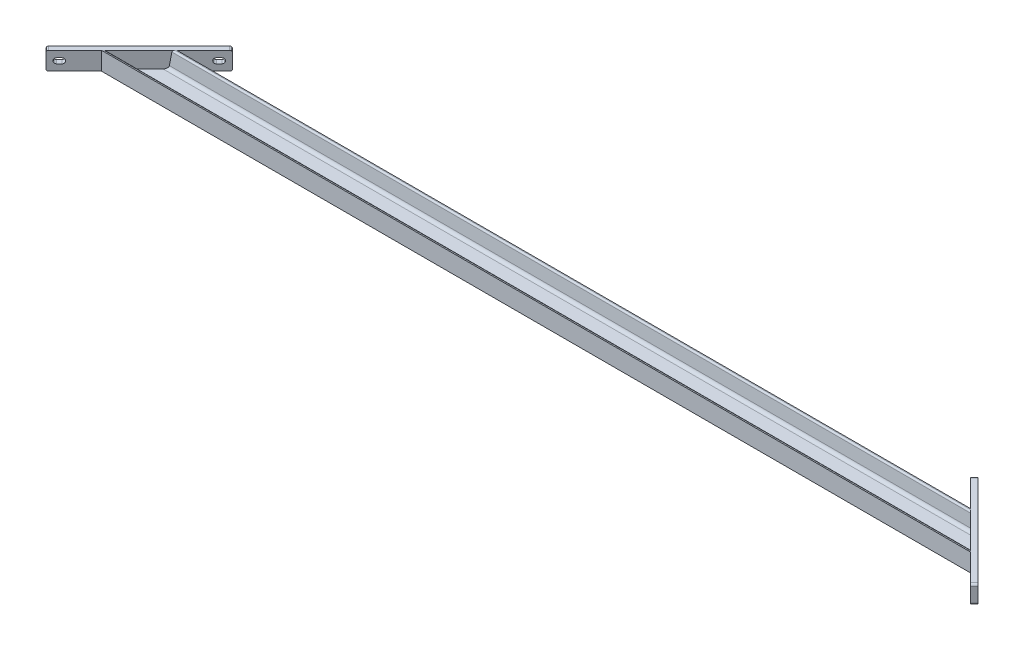
SolidWorks part; units mm, degrees
material "普通碳钢"
ref_plane "Front Plane" through (0, 0, 0) normal (0, 0, 1) x (1, 0, 0)
ref_plane "Top Plane" through (0, 0, 0) normal (0, 1, 0) x (1, 0, 0)
ref_plane "Right Plane" through (0, 0, 0) normal (1, 0, 0) x (0, 0, -1)
other "Configuration Table"
sketch "草图1" plane through (0, 0, 0) normal (0, 0, 1) x (1, 0, 0)
  line L0 (-1153.75, 0) -> (1153.75, 0)
  point P4 (0, 0)
  dimension "D1" = 2307.5
other "Gb／t707-1988 Hot-Rolled Channel 10(1)"
ref_plane "Plane1" through (-1153.75, 0, -50) normal (1, 0, 0) x (0, 1, 0)
sketch "Sketch1" plane through (-1153.75, 0, -50) normal (1, 0, 0) x (0, 1, 0)
  line L0 (48, 100) -> (0, 100)
  line L1 (48, 0) -> (0, 0)
  line L2 (0, 100) -> (0, 0)
  line L3 (-9.5694, 50) -> (49.7414, 50) construction
  line L4 (5.3, 81.6026) -> (5.3, 18.3974)
  line L5 (48, 0) -> (48, 2.4743)
  line L6 (48, 100) -> (48, 97.5257)
  line L7 (12.9115, 9.944) -> (44.239, 6.6513)
  line L17 (12.9115, 90.056) -> (44.239, 93.3487)
  arc A0 (44.239, 93.3487) -> (48, 97.5257) centre (43.8, 97.5257) ccw
  arc A1 (44.239, 6.6513) -> (48, 2.4743) centre (43.8, 2.4743) cw
  arc A2 (5.3, 18.3974) -> (12.9115, 9.944) centre (13.8, 18.3974) ccw
  arc A10 (5.3, 81.6026) -> (12.9115, 90.056) centre (13.8, 81.6026) cw
  point P6 (0, 0)
  point P8 (0, 50)
  point P9 (5.3, 25.8841)
  point P10 (24, 100)
  point P13 (48, 93.744)
  point P14 (26.65, 91.5)
  point P19 (5.3, 50)
sketch "Sketch3" plane through (0, 0, 0) normal (0, -1, 0) x (1, 0, 0)
  line L0 (1153.75, 50) -> (1053.75, -50)
  line L1 (1153.75, -50) -> (-1153.75, -50) construction
  line L2 (1053.75, -50) -> (1153.75, -50)
  line L3 (1153.75, -50) -> (1153.75, 50)
  line L4 (-1153.75, 50) -> (-1153.75, -50)
  line L5 (-1153.75, 50) -> (-1153.75, -50) construction
  line L6 (-1153.75, -50) -> (-1053.75, -50)
  line L7 (-1053.75, -50) -> (-1153.75, 50)
extrude "Cut-Extrude1" cut sketch "Sketch3" against normal through all
sketch "Sketch4" plane through (-551.875, 0, -551.875) normal (-0.7071, 0, -0.7071) x (-0.7071, 0, 0.7071)
  line L0 (851.1798, 48) -> (709.7584, 0) construction
  line L1 (630.4691, 24) -> (930.4691, 24) construction
  line L2 (610.4691, 0) -> (950.4691, 0)
  line L3 (605.4691, 5) -> (605.4691, 43)
  line L4 (610.4691, 48) -> (950.4691, 48)
  line L5 (955.4691, 5) -> (955.4691, 43)
  line L6 (605.4691, 0) -> (955.4691, 48) construction
  line L7 (605.4691, 48) -> (955.4691, 0) construction
  line L8 (925.4691, 24) -> (935.4691, 24) construction
  line L9 (925.4691, 31) -> (935.4691, 31)
  line L12 (925.4691, 17) -> (935.4691, 17)
  line L14 (625.4691, 24) -> (635.4691, 24) construction
  line L15 (625.4691, 31) -> (635.4691, 31)
  line L18 (625.4691, 17) -> (635.4691, 17)
  line L27 (625.4691, 74) -> (635.4691, 74) construction
  line L28 (630.4691, -26) -> (930.4691, -26) construction
  line L29 (630.4691, -26) -> (630.4691, 74) construction
  line L30 (630.4691, 74) -> (930.4691, 74) construction
  line L31 (930.4691, -26) -> (930.4691, 74) construction
  line L32 (630.4691, -26) -> (930.4691, 74) construction
  line L33 (630.4691, 74) -> (930.4691, -26) construction
  line L34 (625.4691, 81) -> (635.4691, 81) construction
  line L35 (625.4691, 67) -> (635.4691, 67) construction
  line L36 (625.4691, -26) -> (635.4691, -26) construction
  line L37 (625.4691, -19) -> (635.4691, -19) construction
  line L38 (625.4691, -33) -> (635.4691, -33) construction
  line L39 (925.4691, 74) -> (935.4691, 74) construction
  line L40 (925.4691, 81) -> (935.4691, 81) construction
  line L41 (925.4691, 67) -> (935.4691, 67) construction
  line L42 (925.4691, -26) -> (935.4691, -26) construction
  line L43 (925.4691, -19) -> (935.4691, -19) construction
  line L44 (925.4691, -33) -> (935.4691, -33) construction
  arc A12 (625.4691, 81) -> (625.4691, 67) centre (625.4691, 74) ccw construction
  arc A13 (635.4691, 67) -> (635.4691, 81) centre (635.4691, 74) ccw construction
  arc A14 (625.4691, -19) -> (625.4691, -33) centre (625.4691, -26) ccw construction
  arc A15 (635.4691, -33) -> (635.4691, -19) centre (635.4691, -26) ccw construction
  arc A16 (925.4691, 81) -> (925.4691, 67) centre (925.4691, 74) ccw construction
  arc A17 (935.4691, 67) -> (935.4691, 81) centre (935.4691, 74) ccw construction
  arc A18 (925.4691, -19) -> (925.4691, -33) centre (925.4691, -26) ccw construction
  arc A19 (935.4691, -33) -> (935.4691, -19) centre (935.4691, -26) ccw construction
  arc A20 (950.4691, 0) -> (955.4691, 5) centre (950.4691, 5) ccw
  arc A21 (950.4691, 48) -> (955.4691, 43) centre (950.4691, 43) cw
  arc A22 (610.4691, 0) -> (605.4691, 5) centre (610.4691, 5) cw
  arc A23 (605.4691, 43) -> (610.4691, 48) centre (610.4691, 43) cw
  arc A24 (925.4691, 31) -> (925.4691, 17) centre (925.4691, 24) ccw
  arc A25 (935.4691, 17) -> (935.4691, 31) centre (935.4691, 24) ccw
  arc A26 (625.4691, 31) -> (625.4691, 17) centre (625.4691, 24) ccw
  arc A27 (635.4691, 17) -> (635.4691, 31) centre (635.4691, 24) ccw
  point P4 (780.4691, 24)
  point P24 (780.4691, 24)
  point P26 (930.4691, 24)
  point P32 (630.4691, 24)
  point P49 (780.4691, 24)
  point P56 (630.4691, 74)
  point P62 (630.4691, -26)
  point P69 (930.4691, 74)
  point P76 (930.4691, -26)
  dimension "D3" = 5
  dimension "D1" = 48
  dimension "D2" = 350
  dimension "D8" = 300
  dimension "D9" = 100
  dimension "D10" = 14
  dimension "D11" = 10
extrude "Boss-Extrude1" add sketch "Sketch4" along normal blind 14 separate body
mirror "Mirror1" about plane through (0, 0, 0) normal (1, 0, 0) of bodies 108
equation "\"RI@Sketch1\"= \"D1@Sketch1\""
equation "\"D3@Sketch1\"=  ( \"BF@Sketch1\" - \"D6@Sketch1\" )  / 2"
